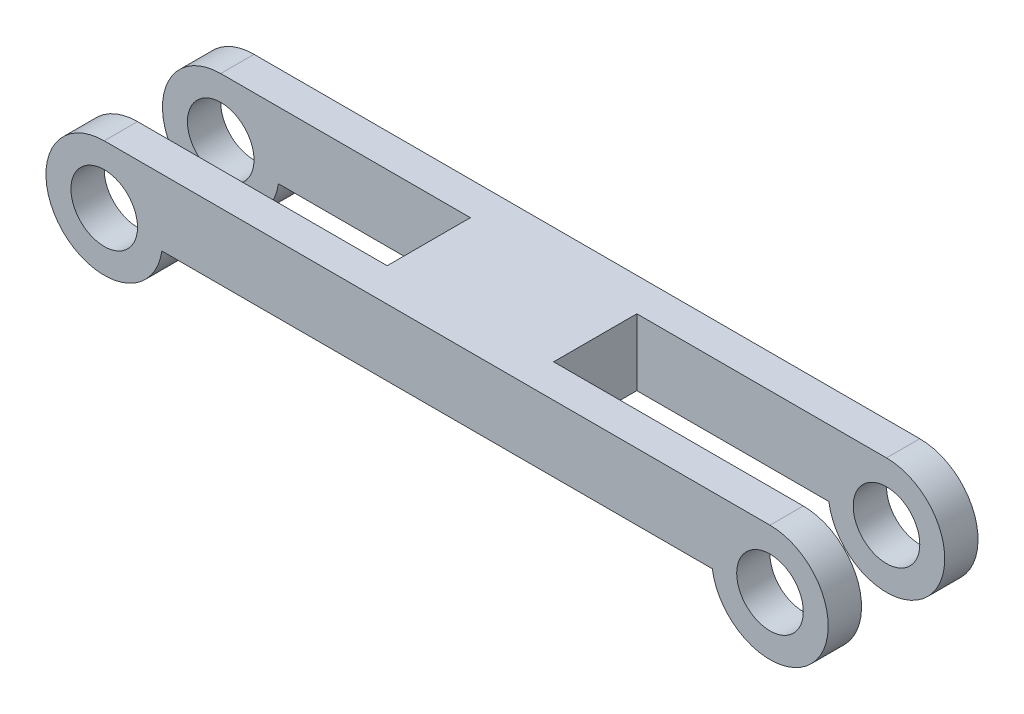
SolidWorks part; units mm, degrees
ref_plane "Front Plane" through (0, 0, 0) normal (0, 0, 1) x (1, 0, 0)
ref_plane "Top Plane" through (0, 0, 0) normal (0, 1, 0) x (1, 0, 0)
ref_plane "Right Plane" through (0, 0, 0) normal (1, 0, 0) x (0, 0, -1)
other "Configuration Table"
sketch "Sketch1" plane through (0, 0, 0) normal (0, 0, 1) x (1, 0, 0)
  line L0 (-20, 0) -> (20, 0)
  line L1 (-16.5359, -4) -> (16.5359, -4)
  circle A0 centre (20, -3.5) radius 2
  circle A1 centre (-20, -3.5) radius 2
  arc A2 (-20, 0) -> (-16.5359, -4) centre (-20, -3.5) ccw
  arc A3 (16.5359, -4) -> (20, 0) centre (20, -3.5) ccw
  point P4 (0, 0)
  dimension "D3" = 4
  dimension "D4" = 4
  dimension "D5" = 7
  dimension "D6" = 7
  dimension "D1" = 3.5
  dimension "D2" = 4
  dimension "D7" = 20
extrude "Boss-Extrude1" add sketch "Sketch1" along normal blind 9
sketch "Sketch2" plane through (0, 0, 0) normal (0, 1, 0) x (1, 0, 0)
  line L0 (-23.5, 0) -> (-23.5, -9) construction
  line L1 (-42, -2) -> (-5, -2)
  line L2 (-42, -2) -> (-42, -7)
  line L3 (-42, -7) -> (-5, -7)
  line L4 (-5, -2) -> (-5, -7)
  line L5 (-23.5, -7) -> (-23.5, -2) construction
  line L6 (-42, -4.5) -> (-5, -4.5) construction
  point P0 (-23.5, -4.5)
  dimension "D1" = 5
  dimension "D2" = 5
extrude "Cut-Extrude1" cut sketch "Sketch2" against normal blind 9
mirror "Mirror1" about plane through (0, 0, 0) normal (1, 0, 0) of "Cut-Extrude1"
